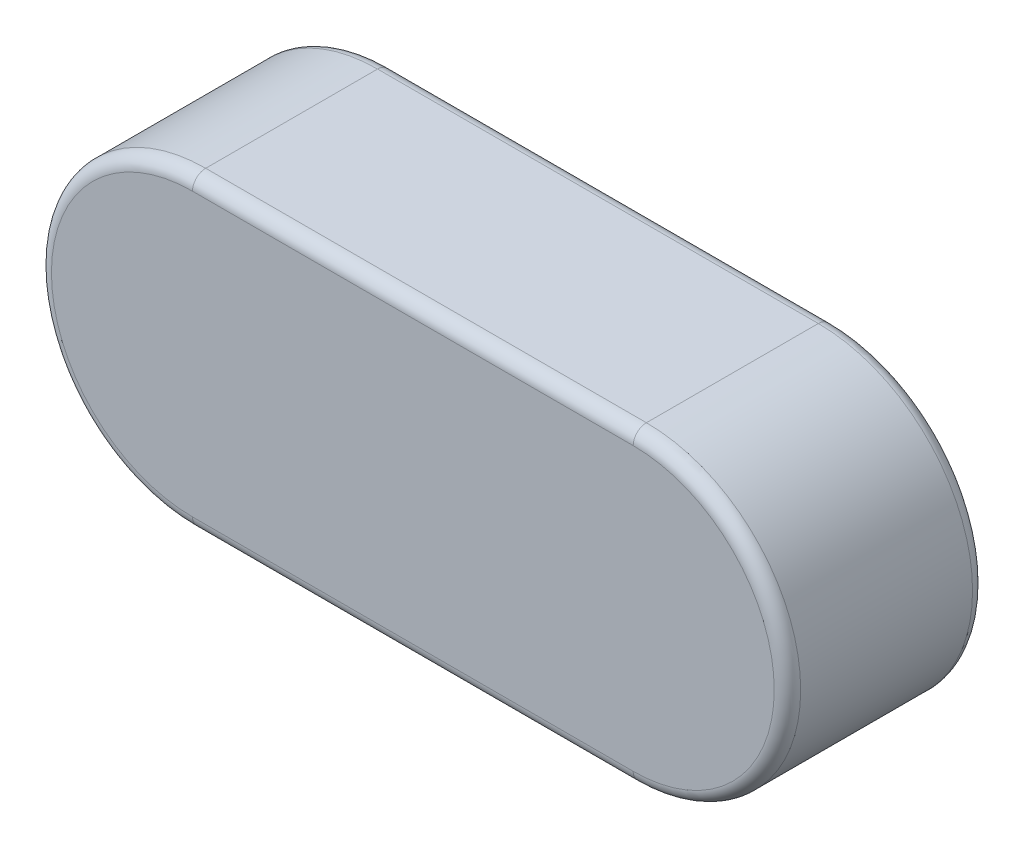
from build123d import *

# Parameters (mm, degrees)
EXTRUDE_524_DEPTH = 9
FILLET_1_R        = 0.6


with BuildPart() as part:
    # 草图1 → Extrude 524 (new body)
    with BuildSketch(Plane.XY):
        with BuildLine():
            Line((-10, 7), (10, 7))
            ThreePointArc((10, 7), (17, 0), (10, -7))
            Line((10, -7), (-10, -7))
            ThreePointArc((-10, -7), (-17, 0), (-10, 7))
        make_face()
    extrude(amount=EXTRUDE_524_DEPTH)

    # 圆角1
    fillet_1_edges = [part.edges().sort_by_distance(p)[0] for p in [
        (17, 0, 9),
        (0, 7, 9),
        (-17, 0, 9),
        (0, 7, 0),
        (17, 0, 0),
        (0, -7, 0),
        (-17, 0, 0),
        (0, -7, 9),
    ]]
    fillet(fillet_1_edges, radius=FILLET_1_R)


solid = part.part
